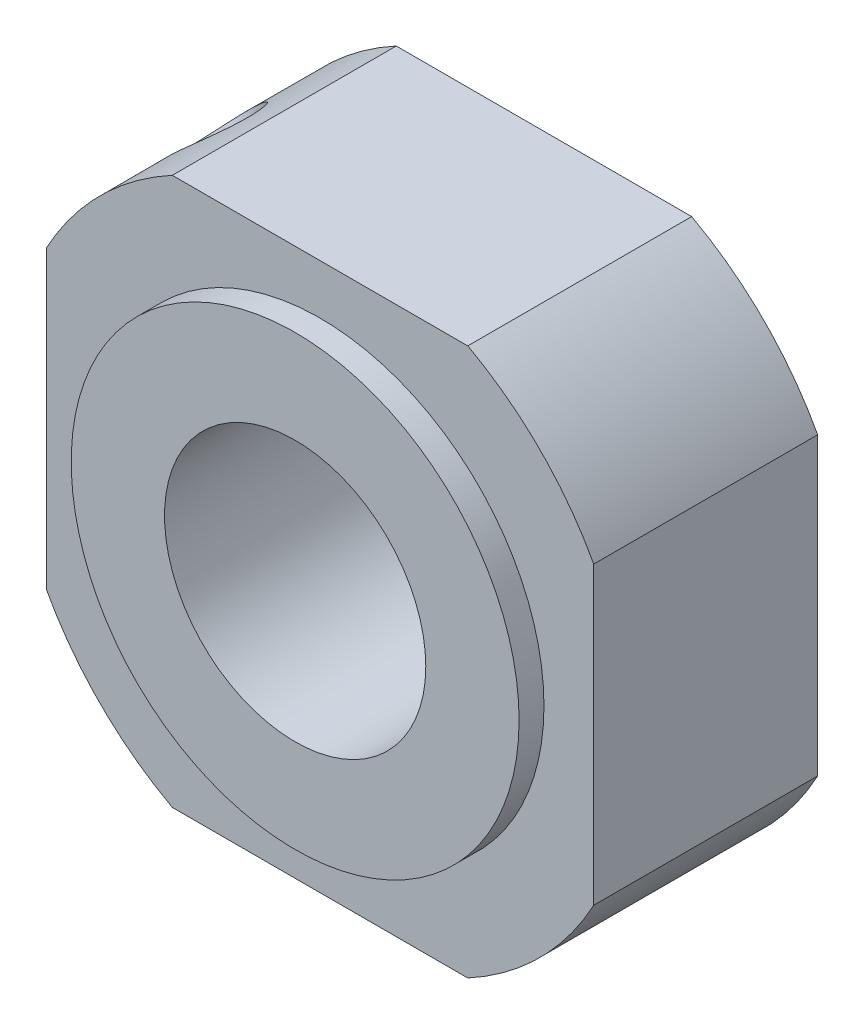
SolidWorks part; units mm, degrees
ref_plane "Front Plane" through (0, 0, 0) normal (0, 0, 1) x (1, 0, 0)
ref_plane "Top Plane" through (0, 0, 0) normal (0, 1, 0) x (1, 0, 0)
ref_plane "Right Plane" through (0, 0, 0) normal (1, 0, 0) x (0, 0, -1)
sketch "Sketch1" plane through (0, 0, 0) normal (0, 0, 1) x (1, 0, 0)
  line L0 (-5.9372, -11) -> (5.9372, -11)
  line L1 (5.9372, 11) -> (-5.9372, 11)
  line L2 (-11, 5.9372) -> (-11, -5.9372)
  line L3 (11, -5.9372) -> (11, 5.9372)
  arc A0 (5.9372, -11) -> (11, -5.9372) centre (0, 0) ccw
  arc A1 (-11, -5.9372) -> (-5.9372, -11) centre (0, 0) ccw
  arc A2 (11, 5.9372) -> (5.9372, 11) centre (0, 0) ccw
  arc A3 (-5.9372, 11) -> (-11, 5.9372) centre (0, 0) ccw
  dimension "D2" = 11
  dimension "D5" = 12.5
  dimension "D1" = 22
  dimension "D3" = 11
  dimension "D4" = 22
extrude "Extrude1" add sketch "Sketch1" along normal blind 10
sketch "Sketch2" plane through (0, 0, 10) normal (0, 0, 1) x (1, 0, 0)
  circle A0 centre (0, 0) radius 9
  dimension "D1" = 18
extrude "Extrude2" cut sketch "Sketch2" against normal blind 1 flip side to cut
hole_wizard "M4x0.7 Tapped Hole1" positions "3DSketch1" profile "Sketch3" tap size "M4x0.7" standard "Ansi Metric"
sketch3d "3DSketch1"
  line L0 (-5.9372, 11, 9) -> (-5.9372, 11, 0) construction
  line L1 (-11, 5.9372, 9) -> (-11, -5.9372, 9) construction
  point P0 (-8.5355, 9.1321, 4.6496)
  dimension "D1" = 3.2
  dimension "D2" = 5
sketch "Sketch3" plane through (-8.5355, 9.1321, 4.6496) normal (0, 0, 1) x (-0.7306, -0.6828, 0)
  line L0 (0, 0) -> (0, 11.0914)
  line L1 (0, 11.0914) -> (1.65, 10.1)
  line L2 (1.65, 10.1) -> (1.65, 0)
  line L5 (1.65, 0) -> (0, 0)
  line L10 (0, 11.0914) -> (-1.65, 10.1) construction
  line L11 (0, -6.35) -> (0, 107.95) construction
  dimension "螺纹孔钻头直径" = 3.3
  dimension "螺纹孔钻头深度" = 10.1
  dimension "导头角度" = 118
cosmetic thread "Cosmetic Thread1" parameters "D1"=6.2129, "D2"=4
hole_wizard "M12x1.5 Tapped Hole1" positions "Sketch5" profile "Sketch4" tap size "M12x1.5" standard "Ansi Metric"
sketch "Sketch5" plane through (0, 0, 10) normal (0, 0, 1) x (1, 0, 0)
  point P0 (0, 0)
sketch "Sketch4" plane through (0, 0, 10) normal (1, 0, 0) x (0, -1, 0)
  line L0 (0, 0) -> (0, 31.6545)
  line L1 (0, 31.6545) -> (5.25, 28.5)
  line L2 (5.25, 28.5) -> (5.25, 0)
  line L5 (5.25, 0) -> (0, 0)
  line L10 (0, 31.6545) -> (-5.25, 28.5) construction
  line L11 (0, -6.35) -> (0, 107.95) construction
  dimension "螺纹孔钻头直径" = 10.5
  dimension "螺纹孔钻头深度" = 28.5
  dimension "导头角度" = 118
cosmetic thread "Cosmetic Thread3" parameters "D1"=10, "D2"=12
